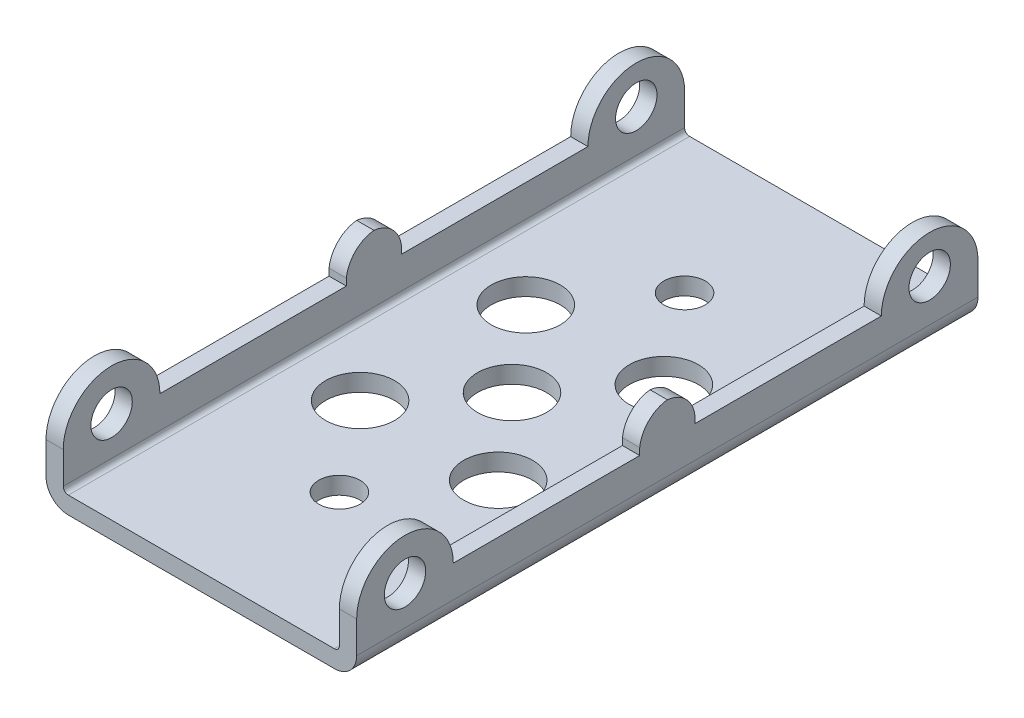
SolidWorks part; units mm, degrees
ref_plane "Front Plane" through (0, 0, 0) normal (0, 0, 1) x (1, 0, 0)
ref_plane "Top Plane" through (0, 0, 0) normal (0, 1, 0) x (1, 0, 0)
ref_plane "Right Plane" through (0, 0, 0) normal (1, 0, 0) x (0, 0, -1)
other "Configuration Table"
ref_plane "Plane1" through (-22.4981, 0, 0) normal (-1, 0, 0) x (0, -1, 0)
sketch "Sketch1" plane through (-22.4981, 0, 0) normal (-1, 0, 0) x (0, -1, 0)
  line L0 (-5.3545, -90) -> (2.5, -90)
  line L1 (2.5, -90) -> (2.5, 0)
  line L2 (2.5, 0) -> (-5.3545, 0)
  line L3 (-5.3545, -14) -> (-5.3545, -41)
  line L4 (-5.3545, -41) -> (-6.3545, -41)
  line L5 (-6.3545, -49) -> (-5.3545, -49)
  line L6 (-5.3545, -49) -> (-5.3545, -76)
  arc A0 (-5.3545, 0) -> (-5.3545, -14) centre (-5.3545, -7) ccw
  arc A1 (-6.3545, -41) -> (-10.3545, -45) centre (-5.8545, -45.5) ccw
  arc A2 (-10.3545, -45) -> (-6.3545, -49) centre (-5.8545, -44.5) ccw
  arc A3 (-5.3545, -76) -> (-5.3545, -90) centre (-5.3545, -83) ccw
extrude "Boss-Extrude1" add sketch "Sketch1" against normal blind 2.5
sketch "Sketch2" plane through (-19.9981, 0, 0) normal (1, 0, 0) x (0, 0, -1)
  line L0 (0, 0) -> (90, 0)
  line L1 (90, 0) -> (90, -2.5)
  line L2 (90, -2.5) -> (0, -2.5)
  line L3 (0, -2.5) -> (0, 0)
extrude "Boss-Extrude2" add sketch "Sketch2" along normal blind 40
sketch "Sketch3" plane through (20.0019, 0, 0) normal (1, 0, 0) x (0, 0, -1)
  line L0 (0, -2.5) -> (0, 5.3508)
  line L1 (14, 5.3508) -> (41, 5.3508)
  line L2 (41, 5.3508) -> (41, 6.3508)
  line L3 (49, 6.3508) -> (49, 5.3508)
  line L4 (49, 5.3508) -> (76, 5.3508)
  line L5 (90, 5.3508) -> (90, -2.5)
  line L6 (90, -2.5) -> (0, -2.5)
  arc A0 (0, 5.3508) -> (14, 5.3508) centre (7, 5.3508) cw
  arc A1 (41, 6.3508) -> (45, 10.3508) centre (45.5, 5.8508) cw
  arc A2 (45, 10.3508) -> (49, 6.3508) centre (44.5, 5.8508) cw
  arc A3 (76, 5.3508) -> (90, 5.3508) centre (83, 5.3508) cw
extrude "Boss-Extrude3" add sketch "Sketch3" along normal blind 2.5
hole_wizard "Ø6.0 (6) Diameter Hole1" positions "Sketch5" profile "Sketch4" hole size "Ø6.0" standard "ANSI Metric"
sketch "Sketch5" plane through (20.0019, 0, 0) normal (-1, 0, 0) x (0, 0, 1)
  point P0 (-83, 6.8508)
  point P1 (-7, 6.3508)
sketch "Sketch4" plane through (20.0019, 6.8508, -83) normal (0, 1, 0) x (0, 0, 1)
  line L0 (0, 0) -> (0, 2.5)
  line L1 (0, 2.5) -> (3, 2.5)
  line L2 (3, 2.5) -> (3, 0)
  line L5 (3, 0) -> (0, 0)
  line L11 (0, -6.35) -> (0, 107.95) construction
  dimension "通孔孔直径" = 6
  dimension "通孔孔深度" = 2.5
hole_wizard "Ø6.0 (6) Diameter Hole2" positions "Sketch7" profile "Sketch6" hole size "Ø6.0" standard "ANSI Metric"
sketch "Sketch7" plane through (-19.9981, 0, 0) normal (1, 0, 0) x (0, 0, -1)
  point P0 (83, 6.8545)
  point P1 (7, 6.3545)
sketch "Sketch6" plane through (-19.9981, 6.8545, -83) normal (0, 1, 0) x (0, 0, -1)
  line L0 (0, 0) -> (0, 2.5)
  line L1 (0, 2.5) -> (3, 2.5)
  line L2 (3, 2.5) -> (3, 0)
  line L5 (3, 0) -> (0, 0)
  line L11 (0, -6.35) -> (0, 107.95) construction
  dimension "通孔孔直径" = 6
  dimension "通孔孔深度" = 2.5
hole_wizard "Ø10.0 (10) Diameter Hole1" positions "Sketch9" profile "Sketch8" hole size "Ø10.0" standard "ANSI Metric"
sketch "Sketch9" plane through (0, 0, 0) normal (0, 1, 0) x (1, 0, 0)
  point P0 (0, 45)
  point P1 (-10, 57)
  point P2 (-10, 33)
  point P3 (10, 33)
  point P4 (10, 57)
sketch "Sketch8" plane through (0, 0, -45) normal (1, 0, 0) x (0, 0, 1)
  line L0 (0, 0) -> (0, 2.5)
  line L1 (0, 2.5) -> (5, 2.5)
  line L2 (5, 2.5) -> (5, 0)
  line L5 (5, 0) -> (0, 0)
  line L11 (0, -6.35) -> (0, 107.95) construction
  dimension "通孔孔直径" = 10
  dimension "通孔孔深度" = 2.5
hole_wizard "Ø6.0 (6) Diameter Hole3" positions "Sketch11" profile "Sketch10" hole size "Ø6.0" standard "ANSI Metric"
sketch "Sketch11" plane through (0, 0, 0) normal (0, 1, 0) x (1, 0, 0)
  point P0 (0, 70)
  point P1 (0, 20)
sketch "Sketch10" plane through (0, 0, -70) normal (1, 0, 0) x (0, 0, 1)
  line L0 (0, 0) -> (0, 2.5)
  line L1 (0, 2.5) -> (3, 2.5)
  line L2 (3, 2.5) -> (3, 0)
  line L5 (3, 0) -> (0, 0)
  line L11 (0, -6.35) -> (0, 107.95) construction
  dimension "通孔孔直径" = 6
  dimension "通孔孔深度" = 2.5
fillet "Fillet1" radius 0.7366 2 edges at (20.0019, 0, -45) (-19.9981, 0, -45)
fillet "Fillet2" radius 3.2366 2 edges at (22.5019, -2.5, -45) (-22.4981, -2.5, -45)
